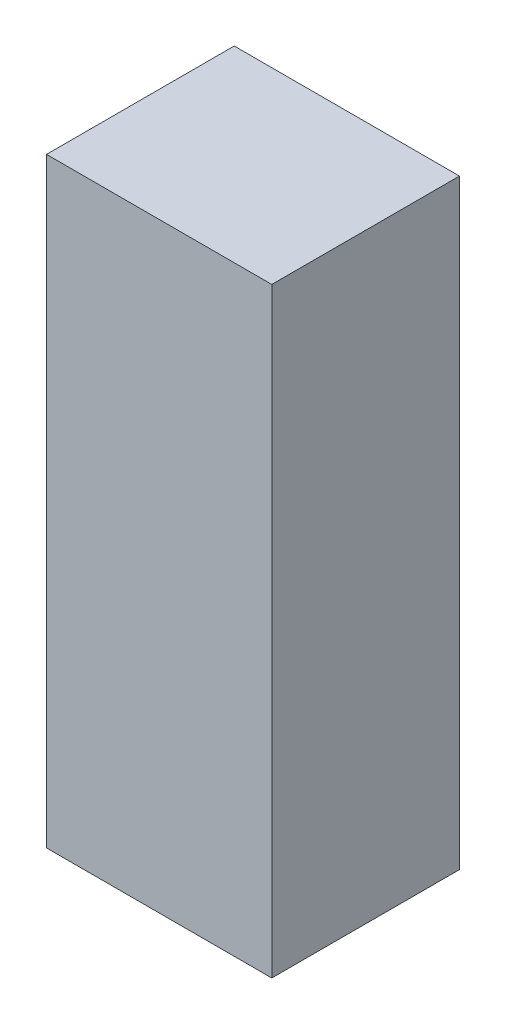
SolidWorks part; units mm, degrees
ref_plane "前视基准面" through (0, 0, 0) normal (0, 0, 1) x (1, 0, 0)
ref_plane "上视基准面" through (0, 0, 0) normal (0, 1, 0) x (1, 0, 0)
ref_plane "右视基准面" through (0, 0, 0) normal (1, 0, 0) x (0, 0, -1)
other "Configuration Table"
sketch "草图1" plane through (0, 0, 0) normal (0, 0, 1) x (1, 0, 0)
  line L0 (-6, -16) -> (6, -16)
  line L1 (6, -16) -> (6, 16)
  line L2 (6, 16) -> (-6, 16)
  line L3 (-6, 16) -> (-6, -16)
  point P0 (0, 0)
  dimension "D1" = 6
  dimension "D2" = 12
  dimension "D3" = 16
  dimension "D4" = 32
extrude "凸台-拉伸1" add sketch "草图1" against normal mid plane 10
